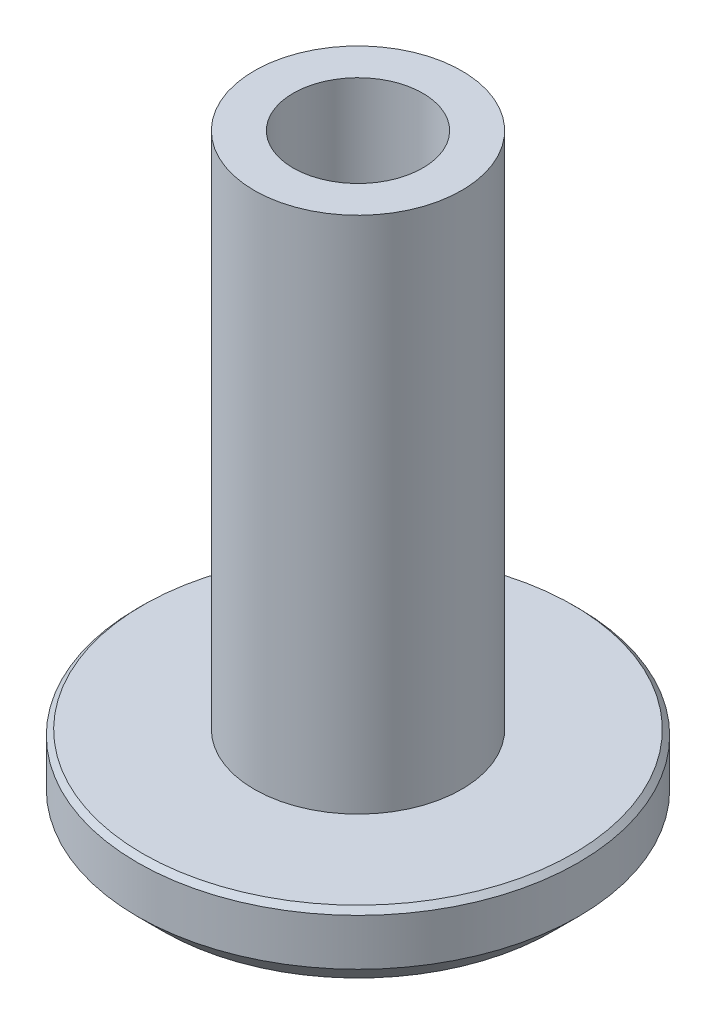
from build123d import *

# Parameters (mm, degrees)
SKETCH_1_R             = 4.25
EXTRUDE_1_DEPTH        = 1.5
SKETCH_2_R             = 2
EXTRUDE_2_DEPTH        = 10
HOLE_WIZARD_M3_1_D     = 2.5
HOLE_WIZARD_M3_1_DEPTH = 8.5
HOLE_WIZARD_M3_1_TIP   = 0.751075774
CUT_EXTRUDE_1_DEPTH    = 1
CHAMFER_1_SIZE         = 0.5
CHAMFER_2_SIZE         = 0.1


with BuildPart() as part:
    # 草图1 → 凸台-拉伸1 (new body)
    with BuildSketch(Plane(origin=(0, 0, 0), x_dir=(1, 0, 0), z_dir=(0, 1, 0))):
        with Locations(Location((0, 0, 0), (0, 0, 270))):
            Circle(SKETCH_1_R)
    extrude(amount=EXTRUDE_1_DEPTH)

    # 草图2 → 凸台-拉伸2 (add)
    with BuildSketch(Plane(origin=(0, 1.5, 0), x_dir=(1, 0, 0), z_dir=(0, 1, 0))):
        with Locations(Location((0, 0, 0), (0, 0, 270))):
            Circle(SKETCH_2_R)
    extrude(amount=EXTRUDE_2_DEPTH)

    # M3 螺纹孔1
    with Locations(Plane(origin=(0, 11.5, 0), x_dir=(1, 0, 0), z_dir=(0, 1, 0))):
        with Locations((0, 0)):
            Hole(HOLE_WIZARD_M3_1_D / 2, depth=HOLE_WIZARD_M3_1_DEPTH)
            with Locations((0, 0, -(HOLE_WIZARD_M3_1_DEPTH + HOLE_WIZARD_M3_1_TIP / 2))):  # 118° drill point
                Cone(0, HOLE_WIZARD_M3_1_D / 2, HOLE_WIZARD_M3_1_TIP, mode=Mode.SUBTRACT)

    # 草图7 → 切除-拉伸1 (cut)
    with BuildSketch(Plane.XZ):
        Polygon((0, 1.443375673), (-1.25, 0.721687836), (-1.25, -0.721687836), (0, -1.443375673), (1.25, -0.721687836), (1.25, 0.721687836), align=None)
    extrude(amount=-CUT_EXTRUDE_1_DEPTH, mode=Mode.SUBTRACT)

    # 倒角1
    chamfer_1_edges = [part.edges().sort_by_distance(p)[0] for p in [
        (0, 0, -4.25),
    ]]
    chamfer(chamfer_1_edges, length=CHAMFER_1_SIZE)

    # 倒角2
    chamfer_2_edges = [part.edges().sort_by_distance(p)[0] for p in [
        (0, 1.5, -4.25),
    ]]
    chamfer(chamfer_2_edges, length=CHAMFER_2_SIZE)


solid = part.part
